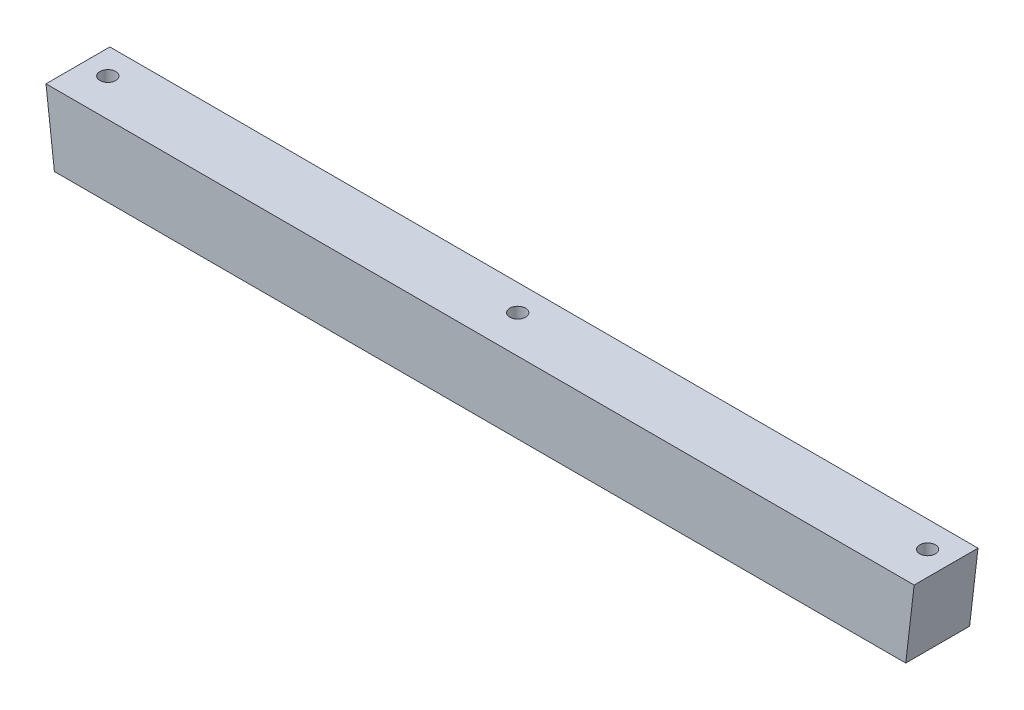
from build123d import *

# Parameters (mm, degrees)
EXTRUDE_1_DEPTH     = 20.25
SKETCH_2_R          = 5
CUT_EXTRUDE_1_DEPTH = 52.5


with BuildPart() as part:
    # 草图1 → 凸台-拉伸1 (new, symmetric)
    with BuildSketch(Plane.XY):
        Polygon((0, 0), (550.66, 0), (545.33, -45.55), (275.33, -45.55), (5.33, -45.55), align=None)
    extrude(amount=EXTRUDE_1_DEPTH, both=True)

    # 草图2 → 切除-拉伸1 (cut)
    with BuildSketch(Plane(origin=(0, 0, 0), x_dir=(1, 0, 0), z_dir=(0, 1, 0))):
        with Locations(Location((535.33, 3.62, 0), (0, 0, 270))):
            Circle(SKETCH_2_R)
        with Locations(Location((275.33, 3.62, 0), (0, 0, 270))):
            Circle(SKETCH_2_R)
        with Locations(Location((15.33, 3.62, 0), (0, 0, 270))):
            Circle(SKETCH_2_R)
    extrude(amount=-CUT_EXTRUDE_1_DEPTH, mode=Mode.SUBTRACT)


solid = part.part
